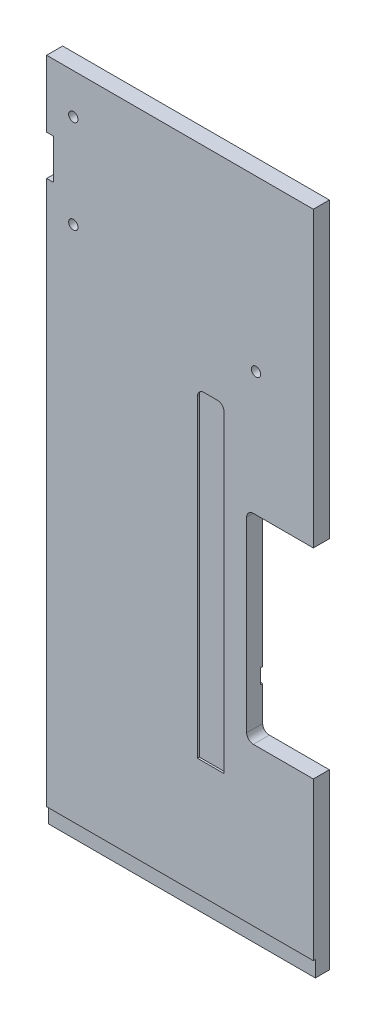
from build123d import *

# Parameters (mm, degrees)
SKETCH_1_W          = 200
SKETCH_1_H          = 500
EXTRUDE_1_DEPTH     = 6
SKETCH_2_W          = 200
SKETCH_2_H          = 11
CUT_EXTRUDE_1_DEPTH = 1.5
CUT_EXTRUDE_2_REACH = 271.526
SKETCH_3_W          = 5
SKETCH_3_H          = 30
CUT_EXTRUDE_3_REACH = 271.526
SKETCH_4_R          = 3.5
SKETCH_5_W          = 20
SKETCH_5_H          = 240
CUT_EXTRUDE_4_DEPTH = 1.5
FILLET_1_R          = 5
CUT_EXTRUDE_5_REACH = 271.526
SKETCH_6_W          = 50
SKETCH_6_H          = 150
FILLET_2_R          = 5
SKETCH_7_W          = 200
SKETCH_7_H          = 12
CUT_EXTRUDE_6_DEPTH = 1.5


with BuildPart() as part:
    # 草图1 → 凸台-拉伸1 (new, symmetric)
    with BuildSketch(Plane.XY):
        Rectangle(SKETCH_1_W, SKETCH_1_H)
    extrude(amount=EXTRUDE_1_DEPTH, both=True)

    # 草图2 → 切除-拉伸1 (cut)
    with BuildSketch(Plane.XY.offset(-6)):
        with Locations((0, -83.5)):
            Rectangle(SKETCH_2_W, SKETCH_2_H)
    extrude(amount=CUT_EXTRUDE_1_DEPTH, mode=Mode.SUBTRACT)

    # 草图3 → 切除-拉伸2 (cut, up to next)
    with BuildSketch(Plane.XY.offset(6), mode=Mode.PRIVATE) as cut_extrude_2_sk1:
        with Locations((-97.5, 185)):
            Rectangle(SKETCH_3_W, SKETCH_3_H)
    cut_extrude_2_tool1 = extrude(cut_extrude_2_sk1.sketch, amount=-CUT_EXTRUDE_2_REACH, mode=Mode.PRIVATE) & part.part
    add(cut_extrude_2_tool1.solids().sort_by_distance((-97.5, 185, 6))[0], mode=Mode.SUBTRACT)

    # 草图4 → 切除-拉伸3 (cut, up to next)
    with BuildSketch(Plane.XY.offset(6), mode=Mode.PRIVATE) as cut_extrude_3_sk1:
        with Locations((-80, 220)):
            Circle(SKETCH_4_R)
    cut_extrude_3_tool1 = extrude(cut_extrude_3_sk1.sketch, amount=-CUT_EXTRUDE_3_REACH, mode=Mode.PRIVATE) & part.part
    # 草图4 → 切除-拉伸3 (cut, up to next)
    with BuildSketch(Plane.XY.offset(6), mode=Mode.PRIVATE) as cut_extrude_3_sk2:
        with Locations((-80, 150)):
            Circle(SKETCH_4_R)
    cut_extrude_3_tool2 = extrude(cut_extrude_3_sk2.sketch, amount=-CUT_EXTRUDE_3_REACH, mode=Mode.PRIVATE) & part.part
    # 草图4 → 切除-拉伸3 (cut, up to next)
    with BuildSketch(Plane.XY.offset(6), mode=Mode.PRIVATE) as cut_extrude_3_sk3:
        with Locations((57, 123)):
            Circle(SKETCH_4_R)
    cut_extrude_3_tool3 = extrude(cut_extrude_3_sk3.sketch, amount=-CUT_EXTRUDE_3_REACH, mode=Mode.PRIVATE) & part.part
    add(cut_extrude_3_tool1.solids().sort_by_distance((-80, 220, 6))[0], mode=Mode.SUBTRACT)
    add(cut_extrude_3_tool2.solids().sort_by_distance((-80, 150, 6))[0], mode=Mode.SUBTRACT)
    add(cut_extrude_3_tool3.solids().sort_by_distance((57, 123, 6))[0], mode=Mode.SUBTRACT)

    # 草图5 → 切除-拉伸4 (cut)
    with BuildSketch(Plane(origin=(0, 0, 6), x_dir=(-1, 0, 0), z_dir=(0, 0, -1))):
        with Locations((-23, -30)):
            Rectangle(SKETCH_5_W, SKETCH_5_H)
    extrude(amount=CUT_EXTRUDE_4_DEPTH, mode=Mode.SUBTRACT)

    # 圆角1
    fillet_1_edges = [part.edges().sort_by_distance(p)[0] for p in [
        (33, 90, 5.25),
        (13, 90, 5.25),
    ]]
    fillet(fillet_1_edges, radius=FILLET_1_R)

    # 草图6 → 切除-拉伸5 (cut, up to next)
    with BuildSketch(Plane(origin=(0, 0, -6), x_dir=(-1, 0, 0), z_dir=(0, 0, -1)), mode=Mode.PRIVATE) as cut_extrude_5_sk1:
        with Locations((-75, -45)):
            Rectangle(SKETCH_6_W, SKETCH_6_H)
    cut_extrude_5_tool1 = extrude(cut_extrude_5_sk1.sketch, amount=-CUT_EXTRUDE_5_REACH, mode=Mode.PRIVATE) & part.part
    add(cut_extrude_5_tool1.solids().sort_by_distance((75, -45, -6))[0], mode=Mode.SUBTRACT)

    # 圆角2
    fillet_2_edges = [part.edges().sort_by_distance(p)[0] for p in [
        (50, 30, 0),
        (50, -120, 0),
    ]]
    fillet(fillet_2_edges, radius=FILLET_2_R)

    # 草图7 → 切除-拉伸6 (cut)
    with BuildSketch(Plane.XY.offset(6)):
        with Locations((0, -244)):
            Rectangle(SKETCH_7_W, SKETCH_7_H)
    extrude(amount=-CUT_EXTRUDE_6_DEPTH, mode=Mode.SUBTRACT)


solid = part.part
